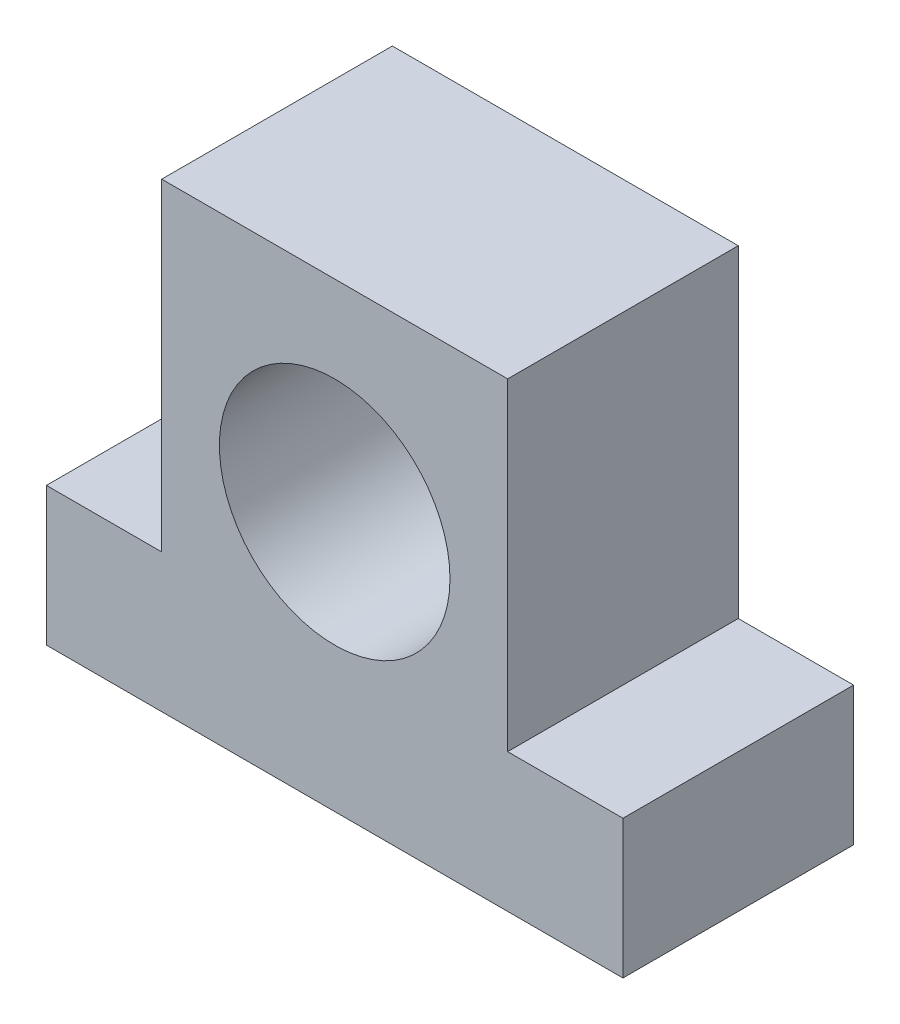
from build123d import *

# Parameters (mm, degrees)
SKETCH_1_W          = 50
SKETCH_1_H          = 40
EXTRUDE_1_DEPTH     = 20
SKETCH_2_R          = 10
CUT_EXTRUDE_1_DEPTH = 38.749172176
SKETCH_3_W          = 10
SKETCH_3_H          = 28
CUT_EXTRUDE_2_DEPTH = 38.749172176


with BuildPart() as part:
    # 草图1 → 凸台-拉伸1 (new body)
    with BuildSketch(Plane.XY):
        Rectangle(SKETCH_1_W, SKETCH_1_H)
    extrude(amount=EXTRUDE_1_DEPTH)

    # 草图2 → 切除-拉伸1 (cut, through all)
    with BuildSketch(Plane.XY.offset(20)):
        with Locations((0, 2.5)):
            Circle(SKETCH_2_R)
    extrude(amount=-CUT_EXTRUDE_1_DEPTH, mode=Mode.SUBTRACT)

    # 草图3 → 切除-拉伸2 (cut, through all)
    with BuildSketch(Plane.XY.offset(20)):
        with Locations((-20, 6)):
            Rectangle(SKETCH_3_W, SKETCH_3_H)
        with Locations((20, 6)):
            Rectangle(SKETCH_3_W, SKETCH_3_H)
    extrude(amount=-CUT_EXTRUDE_2_DEPTH, mode=Mode.SUBTRACT)


solid = part.part
